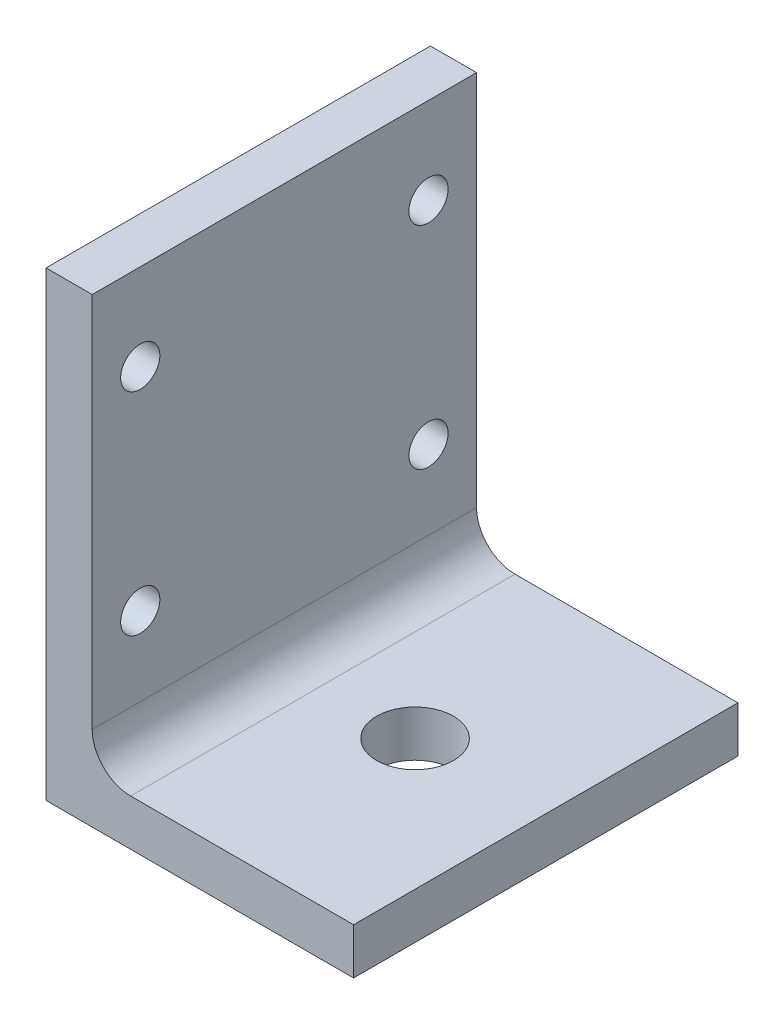
SolidWorks part; units mm, degrees
material "1023 碳钢板 (SS)"
ref_plane "Front Plane" through (0, 0, 0) normal (0, 0, 1) x (1, 0, 0)
ref_plane "Top Plane" through (0, 0, 0) normal (0, 1, 0) x (1, 0, 0)
ref_plane "Right Plane" through (0, 0, 0) normal (1, 0, 0) x (0, 0, -1)
sketch "Sketch1" plane through (0, 0, 0) normal (0, 0, 1) x (1, 0, 0)
  line L0 (0, 0) -> (0, -120)
  line L1 (0, -120) -> (80, -120)
  line L2 (12, 0) -> (12, -98)
  line L3 (22, -108) -> (80, -108)
  line L4 (12, 0) -> (12, -108) construction
  line L5 (12, -108) -> (80, -108) construction
  line L6 (80, -108) -> (80, -120)
  line L7 (12, 0) -> (0, 0)
  arc A0 (12, -98) -> (22, -108) centre (22, -98) ccw
  dimension "D4" = 10
  dimension "D1" = 80
  dimension "D2" = 120
  dimension "D3" = 12
extrude "Boss-Extrude1" add sketch "Sketch1" along normal blind 100 contours L7 L0 L1 L6 L3 A0 L2
sketch "Sketch2" plane through (12, 0, 0) normal (1, 0, 0) x (0, 0, -1)
  line L0 (-100, 0) -> (0, 0) construction
  line L1 (-100, -120) -> (0, -120) construction
  circle A0 centre (-87.5, -22.5) radius 6
  circle A1 centre (-12.5, -22.5) radius 6
  circle A2 centre (-87.5, -77.5) radius 6
  circle A3 centre (-12.5, -77.5) radius 6
  point P14 (-50, 0)
  dimension "D1" = 12
  dimension "D2" = 75
  dimension "D4" = 37.5
  dimension "D5" = 42.5
  dimension "D3" = 55
hole_wizard "M12 Tapped Hole1" positions "Sketch3" profile "Sketch4" tap size "M12" standard "ISO"
sketch "Sketch3" plane through (12, 0, 0) normal (1, 0, 0) x (0, 0, -1)
  point P0 (-87.5, -22.5)
  point P3 (-12.5, -22.5)
  point P6 (-12.5, -77.5)
  point P9 (-87.5, -77.5)
sketch "Sketch4" plane through (12, -22.5, 87.5) normal (0, 1, 0) x (0, 0, -1)
  line L0 (0, 0) -> (0, 32.3144)
  line L1 (0, 32.3144) -> (5.1, 29.25)
  line L2 (5.1, 29.25) -> (5.1, 0)
  line L5 (5.1, 0) -> (0, 0)
  line L10 (0, 32.3144) -> (-5.1, 29.25) construction
  line L11 (0, -6.35) -> (0, 107.95) construction
  dimension "螺纹孔钻头直径" = 10.2
  dimension "螺纹孔钻头深度" = 29.25
  dimension "导头角度" = 118
cosmetic thread "Hole Thread Line 1" parameters "D1"=24, "D2"=12
cosmetic thread "Hole Thread Line 2" parameters "D1"=24, "D2"=12
cosmetic thread "Hole Thread Line 3" parameters "D1"=24, "D2"=12
cosmetic thread "Hole Thread Line 4" parameters "D1"=24, "D2"=12
sketch "Sketch5" plane through (0, -108, 0) normal (0, 1, 0) x (1, 0, 0)
  line L0 (80, -100) -> (80, 0) construction
  circle A0 centre (46, -50) radius 10
  point P5 (80, -50)
  dimension "D1" = 20
  dimension "D2" = 34
extrude "Cut-Extrude1" cut sketch "Sketch5" against normal blind 100
